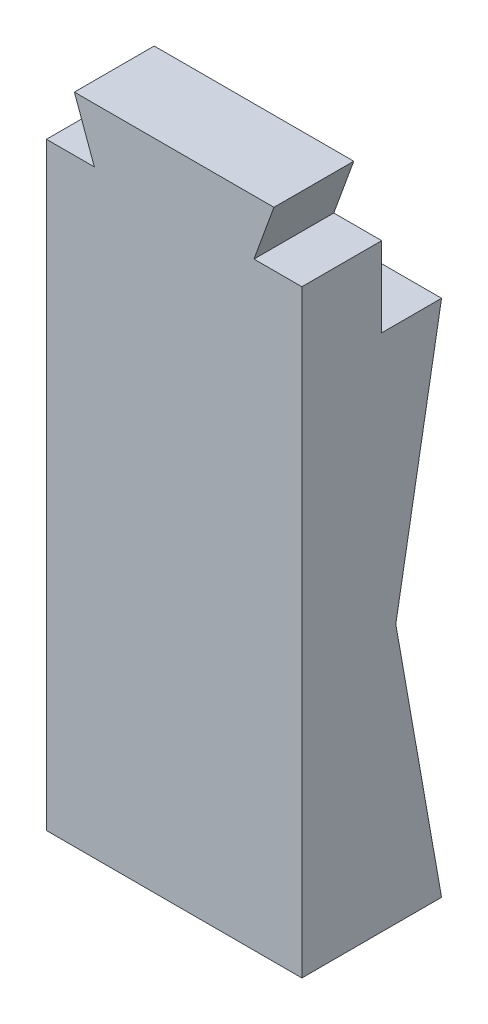
SolidWorks part; units mm, degrees
material "普通碳钢"
ref_plane "Front Plane" through (0, 0, 0) normal (0, 0, 1) x (1, 0, 0)
ref_plane "Top Plane" through (0, 0, 0) normal (0, 1, 0) x (1, 0, 0)
ref_plane "Right Plane" through (0, 0, 0) normal (1, 0, 0) x (0, 0, -1)
sketch "Sketch1" plane through (0, 0, 0) normal (0, 0, 1) x (1, 0, 0)
  line L0 (-27.2622, -0.7809) -> (-27.2622, -150.7809)
  line L1 (36.7378, -0.7809) -> (36.7378, -150.7809)
  line L2 (36.7378, -0.7809) -> (24.7378, -0.7809)
  line L3 (24.7378, -0.7809) -> (29.7378, 12.9565)
  line L4 (29.7378, 12.9565) -> (-20.2622, 12.9565)
  line L5 (-20.2622, 12.9565) -> (-15.2622, -0.7809)
  line L6 (-15.2622, -0.7809) -> (-27.2622, -0.7809)
  line L7 (36.7378, -150.7809) -> (-27.2622, -150.7809)
  dimension "D1" = 150
  dimension "D2" = 70
  dimension "D3" = 50
  dimension "D4" = 70
  dimension "D5" = 12
  dimension "D6" = 12
  dimension "D7" = 64
extrude "Boss-Extrude1" add sketch "Sketch1" along normal blind 20
sketch "Sketch2" plane through (36.7378, 0, 0) normal (1, 0, 0) x (0, 0, -1)
  line L0 (0, -150.7809) -> (15, -150.7809)
  line L1 (15, -150.7809) -> (3.5387, -85.7837)
  line L2 (3.5387, -85.7837) -> (15, -20.7809)
  line L3 (15, -20.7809) -> (0, -20.7809)
  line L5 (0, -20.7809) -> (0, -150.7809)
  dimension "D1" = 15
  dimension "D2" = 15
  dimension "D3" = 160
  dimension "D4" = 66
  dimension "D5" = 130
extrude "Boss-Extrude2" add sketch "Sketch2" against normal blind 64
